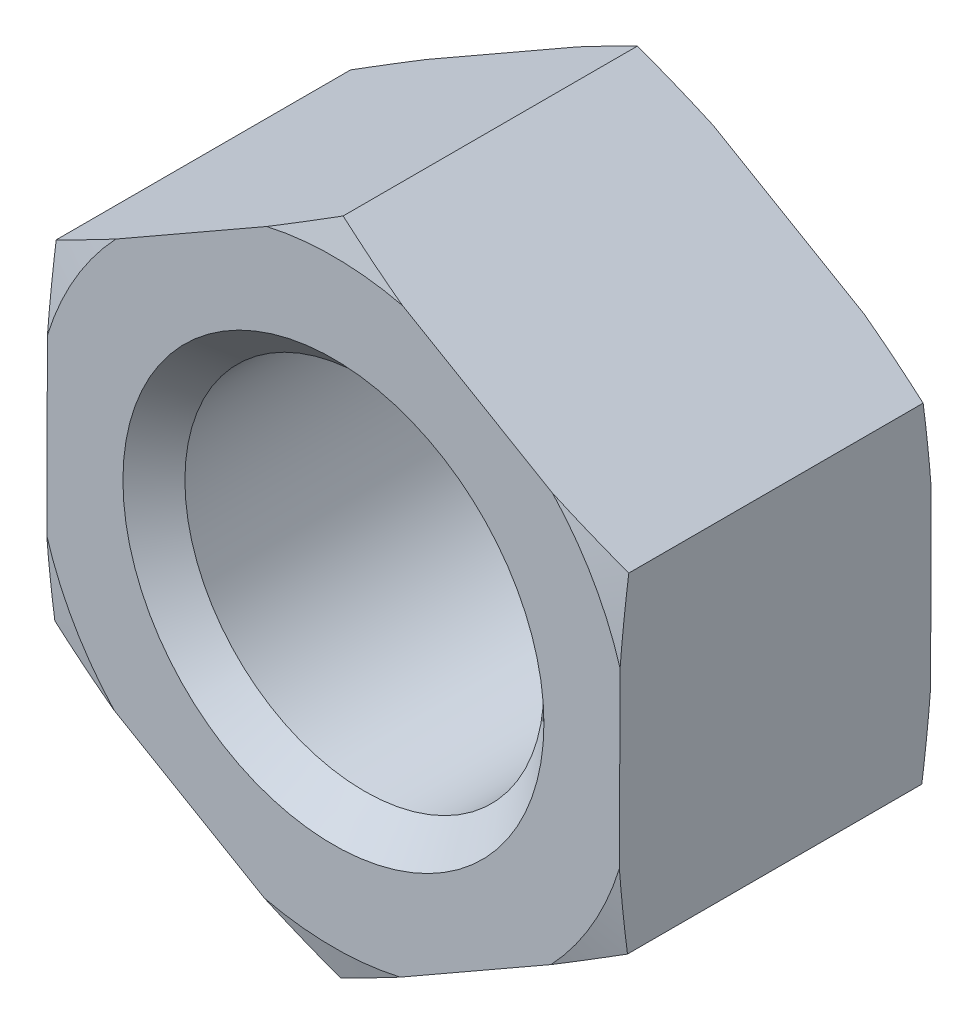
SolidWorks part; units mm, degrees
material "6"
ref_plane "Plane1" through (0, 0, 0) normal (0, 0, 1) x (1, 0, 0)
ref_plane "Plane2" through (0, 0, 0) normal (0, 1, 0) x (1, 0, 0)
ref_plane "Plane3" through (0, 0, 0) normal (1, 0, 0) x (0, 0, -1)
sketch "Dimension sketch" plane through (0, 0, 0) normal (0, 0, 1) x (1, 0, 0)
  line L0 (0, 0) -> (30.6749, 0)
  line L1 (30.6749, 0) -> (37.4249, 0)
  line L2 (37.4249, 0) -> (46.3249, 0)
  line L3 (-5.7143, 0) -> (0, 0)
  point P3 (6, 0)
  point P4 (1.5, 0)
  point P5 (11.05, 0)
  point P6 (5.2, 0)
  point P7 (6.4, 0)
  point P8 (10, 0)
  dimension "D1" = 5.7143
  dimension "D" = 6
  dimension "P" = 1.5
  dimension "e" = 11.05
  dimension "m" = 5.2
  dimension "mw" = 6.4
  dimension "s" = 10
  dimension "da" = 6.75
  dimension "dw" = 8.9
sketch "Sketch1" plane through (0, 0, 0) normal (0, 0, 1) x (1, 0, 0)
  line L0 (-26.8088, 0) -> (37.1748, 0) construction
  line L1 (0, 25.0215) -> (0, -25.0215) construction
  line L3 (0.0217, 5.525) -> (-4.7739, 2.7813)
  line L4 (-4.7739, 2.7813) -> (-4.7956, -2.7437)
  line L5 (-4.7956, -2.7437) -> (-0.0217, -5.525)
  line L6 (-0.0217, -5.525) -> (4.7739, -2.7813)
  line L7 (4.7739, -2.7813) -> (4.7956, 2.7437)
  line L8 (4.7956, 2.7437) -> (0.0217, 5.525)
  circle A0 centre (0, 0) radius 4.7848 construction
  circle A1 centre (0, 0) radius 3
  dimension "D" = 6
  dimension "e" = 11.05
extrude "Base-Extrude" add sketch "Sketch1" along normal blind 5.2
cosmetic thread "Cosmetic Thread1"
chamfer "Chamfer1" distance 0.5179 angle 45 2 edges at (3, 0, 0) (3, 0, 5.2)
sketch "Sketch2" plane through (0, 0, 0) normal (0, 0, -1) x (-1, 0, 0)
  circle A0 centre (0, 0) radius 5
  circle A1 centre (0, 0) radius 3 construction
  dimension "s" = 10
extrude "Cut-Extrude1" cut sketch "Sketch2" against normal through all draft 75 flip side to cut
sketch "Sketch3" plane through (0, 0, 5.2) normal (0, 0, 1) x (1, 0, 0)
  circle A0 centre (0, 0) radius 5
  dimension "D1" = 10
extrude "Cut-Extrude2" cut sketch "Sketch3" against normal through all draft 75 flip side to cut
